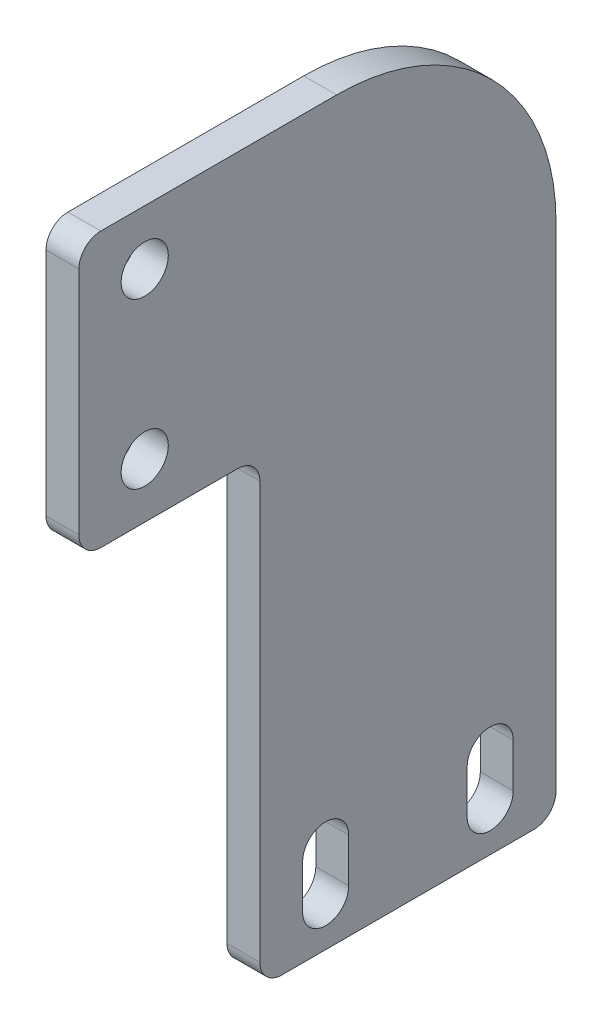
from build123d import *

# Parameters (mm, degrees)
EXTRUDE_1_DEPTH             = 3
EXTRUDE_2_DEPTH             = 3
CUT_EXTRUDE_1_DEPTH         = 3
FILLET_2_R                  = 2
HOLE_WIZARD_4_3_4_3_1_D     = 4.3
HOLE_WIZARD_4_3_4_3_1_DEPTH = 10.1
HOLE_WIZARD_4_3_4_3_1_TIP   = 1.291850331
EXTRUDE_3_DEPTH             = 3
PATTERN_LINEAR_1_COUNT      = 2
PATTERN_LINEAR_1_PITCH      = 24
SKETCH_8_W                  = 24.221203915
SKETCH_8_H                  = 43.975746473
CUT_EXTRUDE_2_DEPTH         = 10
SKETCH_9_W                  = 8.594531195
SKETCH_9_H                  = 29.155429328
CUT_EXTRUDE_3_DEPTH         = 10
FILLET_3_R                  = 2
FILLET_4_R                  = 20


with BuildPart() as part:
    # 草图1 → 凸台-拉伸1 (new body)
    with BuildSketch(Plane(origin=(0, 0, 0), x_dir=(0, 0, -1), z_dir=(1, 0, 0))):
        Polygon((-12.5, 6), (-6, 6), (-6, 61), (6, 61), (6, 6), (12.5, 6), (12.5, -6), (-12.5, -6), align=None)
    extrude(amount=EXTRUDE_1_DEPTH)

    # 草图2 → 凸台-拉伸2 (add)
    with BuildSketch(Plane.ZY):
        Polygon((-6, 61), (-12.5, 6), (12.5, 6), (6, 61), align=None)
    extrude(amount=-EXTRUDE_2_DEPTH)

    # 草图3 → 切除-拉伸1 (cut)
    with BuildSketch(Plane.ZY):
        with BuildLine():
            Line((-5.4, 2), (-5.4, -2))
            ThreePointArc((-5.4, -2), (-7.5, -4.1), (-9.6, -2))
            Line((-9.6, -2), (-9.6, 2))
            ThreePointArc((-9.6, 2), (-7.5, 4.1), (-5.4, 2))
        make_face()
        with BuildLine():
            Line((5.4, 2), (5.4, -2))
            ThreePointArc((5.4, -2), (7.5, -4.1), (9.6, -2))
            Line((9.6, -2), (9.6, 2))
            ThreePointArc((9.6, 2), (7.5, 4.1), (5.4, 2))
        make_face()
    cut_extrude_1 = extrude(amount=-CUT_EXTRUDE_1_DEPTH, mode=Mode.SUBTRACT)

    # 圆角2
    fillet_2_edges = [part.edges().sort_by_distance(p)[0] for p in [
        (1.5, -6, -12.5),
        (1.5, -6, 12.5),
    ]]
    fillet(fillet_2_edges, radius=FILLET_2_R)

    # Ø4.3 (4.3) 直径孔1
    with Locations(Plane.ZY):
        with Locations((0, 56), (0, 41)):
            Hole(HOLE_WIZARD_4_3_4_3_1_D / 2, depth=HOLE_WIZARD_4_3_4_3_1_DEPTH)
            with Locations((0, 0, -(HOLE_WIZARD_4_3_4_3_1_DEPTH + HOLE_WIZARD_4_3_4_3_1_TIP / 2))):  # 118° drill point
                Cone(0, HOLE_WIZARD_4_3_4_3_1_D / 2, HOLE_WIZARD_4_3_4_3_1_TIP, mode=Mode.SUBTRACT)

    # 草图7 → 凸台-拉伸3 (add)
    with BuildSketch(Plane.ZY):
        Polygon((-3.566854944, 61), (-37.5, 61), (-37.5, -6), (-10.5, -6), (-10.5, 36), (-3.566854944, 36), align=None)
    extrude(amount=-EXTRUDE_3_DEPTH)

    # 阵列(线性)1: 切除-拉伸1 ×2
    with Locations(*[(0, 0, -i * PATTERN_LINEAR_1_PITCH) for i in range(1, PATTERN_LINEAR_1_COUNT)]):
        add(cut_extrude_1, mode=Mode.SUBTRACT)

    # 草图8 → 切除-拉伸2 (cut)
    with BuildSketch(Plane.ZY):
        with Locations((1.610601958, 14.012126763)):
            Rectangle(SKETCH_8_W, SKETCH_8_H)
    extrude(amount=-CUT_EXTRUDE_2_DEPTH, mode=Mode.SUBTRACT)

    # 草图9 → 切除-拉伸3 (cut)
    with BuildSketch(Plane.ZY):
        with Locations((10.297265598, 46.422285336)):
            Rectangle(SKETCH_9_W, SKETCH_9_H)
    extrude(amount=-CUT_EXTRUDE_3_DEPTH, mode=Mode.SUBTRACT)

    # 圆角3
    fillet_3_edges = [part.edges().sort_by_distance(p)[0] for p in [
        (1.5, -6, -37.5),
        (1.5, 36, -10.5),
        (1.5, 61, 6),
        (1.5, -6, -10.5),
        (1.5, 36, 6),
    ]]
    fillet(fillet_3_edges, radius=FILLET_3_R)

    # 圆角4
    fillet_4_edges = [part.edges().sort_by_distance(p)[0] for p in [
        (1.5, 61, -37.5),
    ]]
    fillet(fillet_4_edges, radius=FILLET_4_R)


solid = part.part
